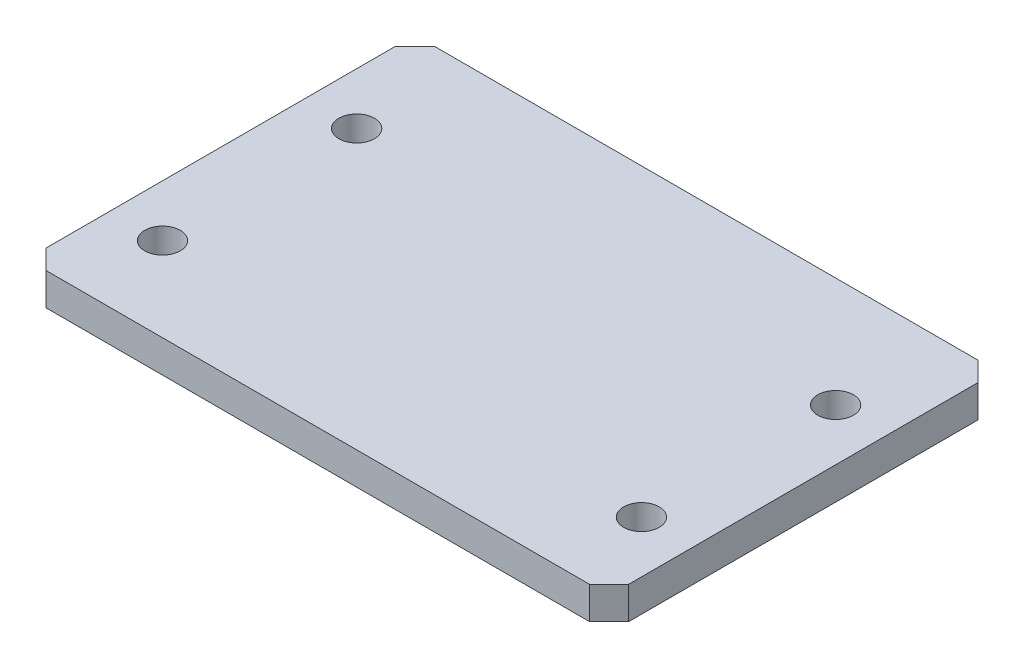
from build123d import *

# Parameters (mm, degrees)
SKETCH_1_W          = 90
SKETCH_1_H          = 60
EXTRUDE_1_DEPTH     = 5
CHAMFER_1_SIZE      = 3
SKETCH_2_R          = 2.75
CUT_EXTRUDE_1_DEPTH = 10


with BuildPart() as part:
    # 草图1 → 凸台-拉伸1 (new body)
    with BuildSketch(Plane(origin=(0, 0, 0), x_dir=(1, 0, 0), z_dir=(0, 1, 0))):
        Rectangle(SKETCH_1_W, SKETCH_1_H)
    extrude(amount=EXTRUDE_1_DEPTH)

    # 倒角1
    chamfer_1_edges = [part.edges().sort_by_distance(p)[0] for p in [
        (45, 2.5, 30),
        (-45, 2.5, 30),
        (-45, 2.5, -30),
        (45, 2.5, -30),
    ]]
    chamfer(chamfer_1_edges, length=CHAMFER_1_SIZE)

    # 草图2 → 切除-拉伸1 (cut)
    with BuildSketch(Plane(origin=(0, 5, 0), x_dir=(1, 0, 0), z_dir=(0, 1, 0))):
        with Locations(Location((37, -17, 0), (0, 0, 270))):
            Circle(SKETCH_2_R)
        with Locations(Location((-37, -17, 0), (0, 0, 270))):
            Circle(SKETCH_2_R)
        with Locations(Location((37, 13, 0), (0, 0, 270))):
            Circle(SKETCH_2_R)
        with Locations(Location((-37, 13, 0), (0, 0, 270))):
            Circle(SKETCH_2_R)
    extrude(amount=-CUT_EXTRUDE_1_DEPTH, mode=Mode.SUBTRACT)


solid = part.part
